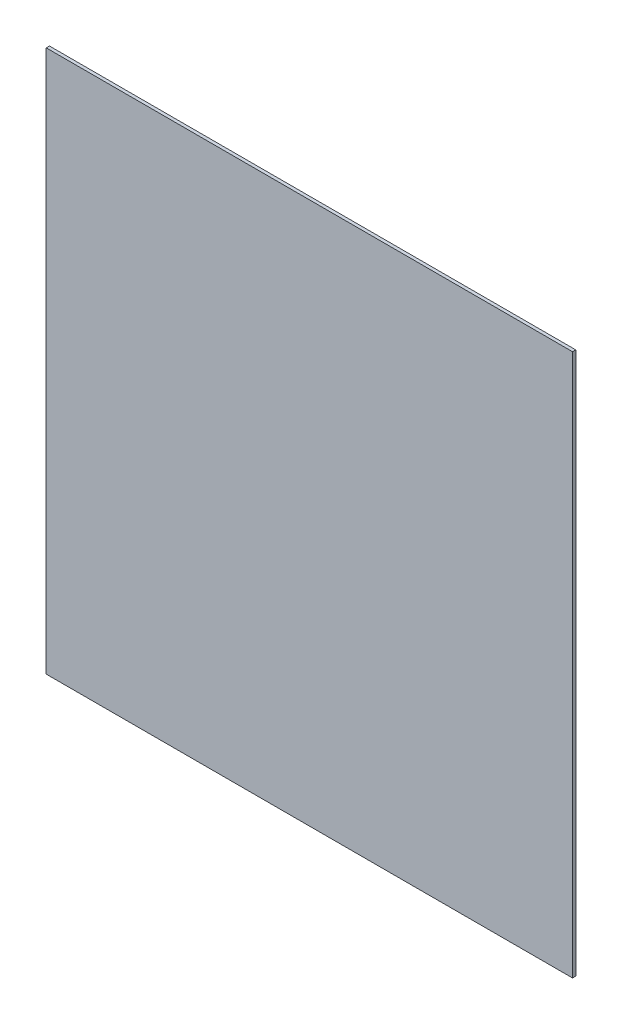
from build123d import *

# Parameters (mm, degrees)
SKETCH_1_W      = 817
SKETCH_1_H      = 842
EXTRUDE_1_DEPTH = 5


with BuildPart() as part:
    # 草图1 → 凸台-拉伸1 (new body)
    with BuildSketch(Plane.XY):
        Rectangle(SKETCH_1_W, SKETCH_1_H)
    extrude(amount=EXTRUDE_1_DEPTH)


solid = part.part
